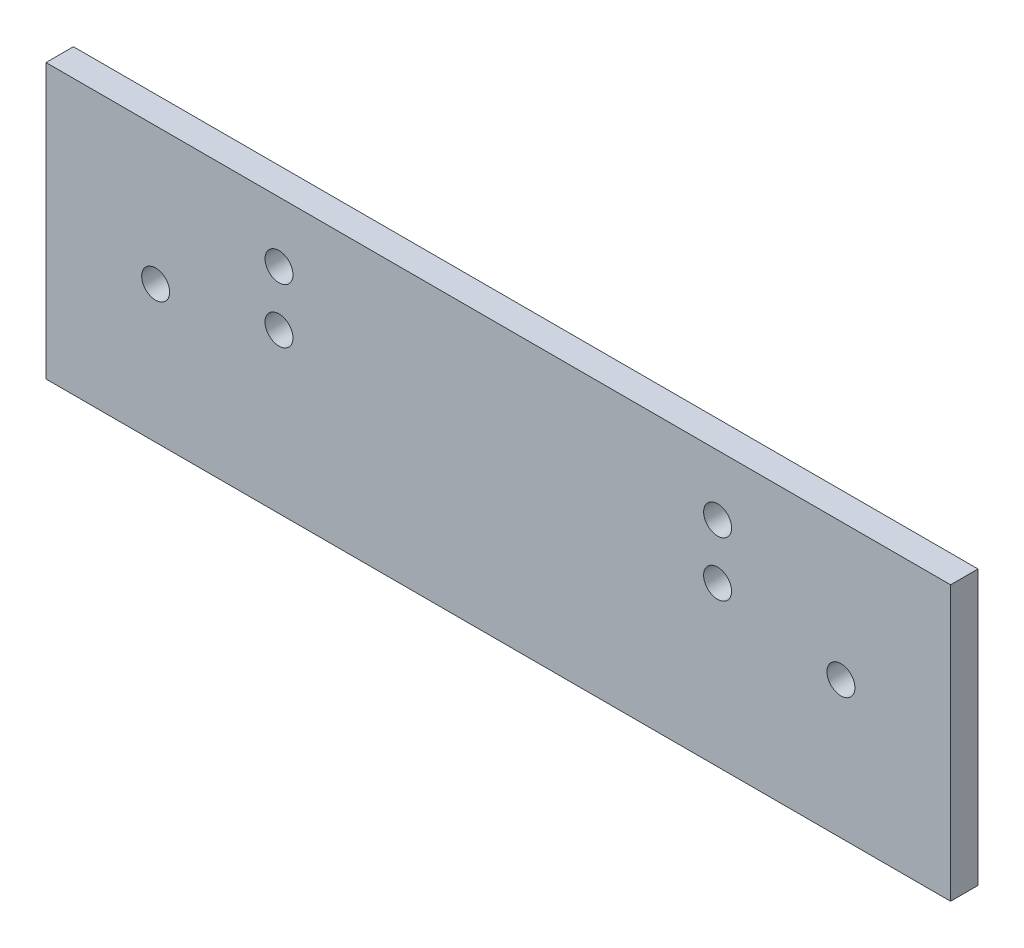
from build123d import *

# Parameters (mm, degrees)
SKETCH1_W              = 330
SKETCH1_H              = 100
BOSS_EXTRUDE1_DEPTH    = 10
M12_TAPPED_HOLE1_D     = 10.2
M12_TAPPED_HOLE1_DEPTH = 29.25
M12_TAPPED_HOLE1_TIP   = 3.064389157


with BuildPart() as part:
    # Sketch1 → Boss-Extrude1 (new body)
    with BuildSketch(Plane.XY):
        Rectangle(SKETCH1_W, SKETCH1_H)
    extrude(amount=BOSS_EXTRUDE1_DEPTH)

    # M12 Tapped Hole1
    with Locations(Plane.XY.offset(10)):
        with Locations((-125, 0), (-80, 8), (-80, 28), (80, 28), (80, 8), (125, 0)):
            Hole(M12_TAPPED_HOLE1_D / 2, depth=M12_TAPPED_HOLE1_DEPTH)
            with Locations((0, 0, -(M12_TAPPED_HOLE1_DEPTH + M12_TAPPED_HOLE1_TIP / 2))):  # 118° drill point
                Cone(0, M12_TAPPED_HOLE1_D / 2, M12_TAPPED_HOLE1_TIP, mode=Mode.SUBTRACT)


solid = part.part
